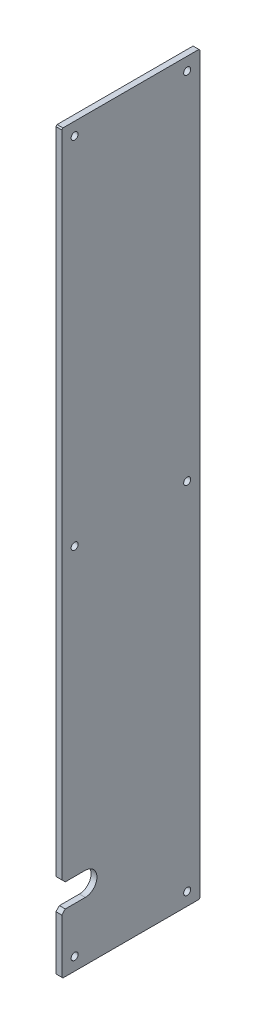
SolidWorks part; units mm, degrees
material "PC(透明)"
ref_plane "前基準面" through (0, 0, 0) normal (0, 0, 1) x (1, 0, 0)
ref_plane "上基準面" through (0, 0, 0) normal (0, 1, 0) x (1, 0, 0)
ref_plane "右基準面" through (0, 0, 0) normal (1, 0, 0) x (0, 0, -1)
sketch "草图1" plane through (0, 0, 0) normal (1, 0, 0) x (0, 0, -1)
  line L1 (59, 314) -> (-59, 314)
  line L2 (59, 314) -> (59, -314)
  line L3 (59, -314) -> (-59, -314)
  line L4 (-59, 314) -> (-59, -314)
  line L5 (59, 314) -> (-59, -314) construction
  line L6 (59, -314) -> (-59, 314) construction
  point P0 (0, 0)
  dimension "D1" = 118
  dimension "D2" = 628
extrude "凸台-拉伸1" add sketch "草图1" along normal blind 5
chamfer "倒角1" distance 1 angle 45 4 edges at (2.5, -314, -59) (2.5, -314, 59) (2.5, 314, -59) (2.5, 314, 59)
sketch "草图2" plane through (0, 0, 0) normal (-1, 0, 0) x (0, 0, 1)
  line L0 (-59, -313) -> (-59, 313) construction
  line L1 (-58, 314) -> (58, 314) construction
  line L2 (58.8862, 0) -> (0, 0) construction
  line L3 (0, 0) -> (0, 69.8386) construction
  line L5 (48, -303) -> (-48, -303) construction
  line L6 (48, -303) -> (48, 303) construction
  line L7 (48, 303) -> (-48, 303) construction
  line L8 (-48, -303) -> (-48, 303) construction
  line L9 (48, -303) -> (-48, 303) construction
  line L10 (48, 303) -> (-48, -303) construction
  circle A0 centre (-48, 303) radius 3
  circle A1 centre (-48, -303) radius 3
  circle A2 centre (48, -303) radius 3
  circle A3 centre (48, 303) radius 3
  circle A8 centre (48, 0) radius 3
  circle A9 centre (-48, 0) radius 3
  dimension "D1" = 6
  dimension "D2" = 11
  dimension "D3" = 11
extrude "切除-拉伸1" cut sketch "草图2" against normal through all
sketch "草图3" plane through (5, 0, 0) normal (1, 0, 0) x (0, 0, -1)
  line L0 (-39, -254) -> (-59, -254) construction
  line L2 (-39, -264) -> (-59, -264)
  line L3 (-39, -244) -> (-59, -244)
  line L4 (-58, -314) -> (58, -314) construction
  line L5 (-59, 313) -> (-59, -313) construction
  arc A0 (-39, -264) -> (-39, -244) centre (-39, -254) ccw
  arc A1 (-59, -244) -> (-59, -264) centre (-59, -254) ccw
  point P4 (-49, -254)
  dimension "D1" = 20
  dimension "D2" = 60
  dimension "D3" = 20
extrude "切除-拉伸2" cut sketch "草图3" against normal through all
chamfer "倒角2" distance 3 angle 45 2 edges at (2.5, -264, 59) (2.5, -244, 59)
